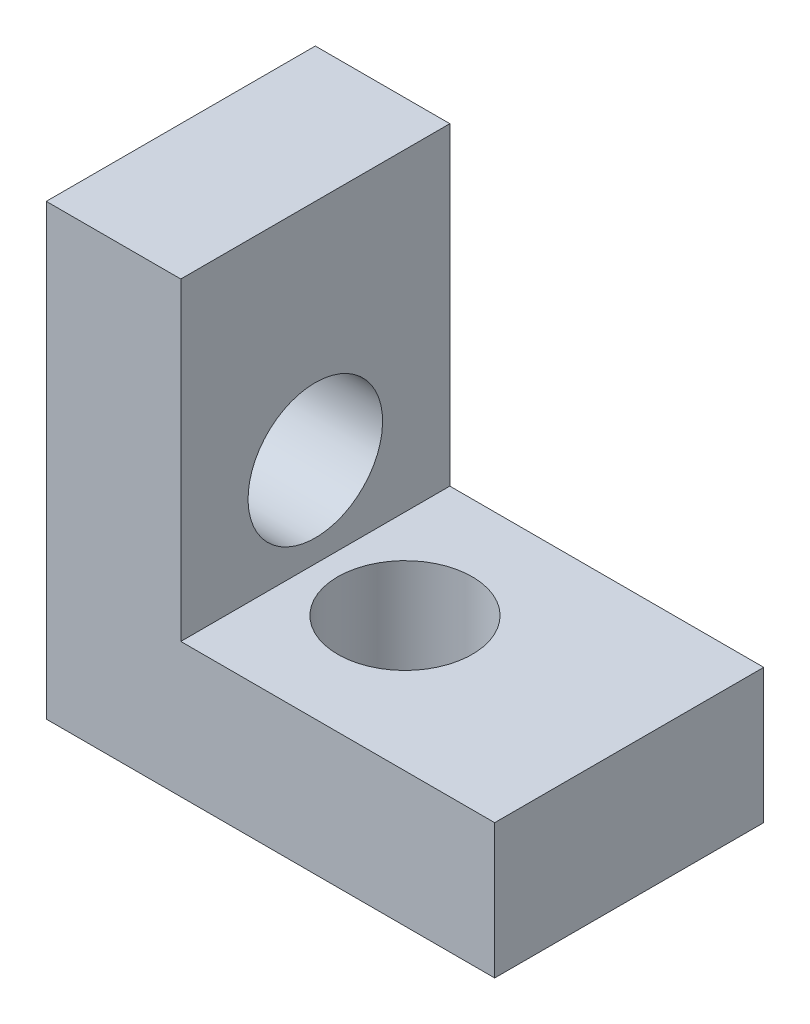
from build123d import *

# Parameters (mm, degrees)
EXTRUDE_4_DEPTH     = 6
SKETCH_7_R          = 1.5
CUT_EXTRUDE_3_DEPTH = 14.601470509
SKETCH_8_R          = 1.5
CUT_EXTRUDE_4_DEPTH = 14.601470509


with BuildPart() as part:
    # 草图6 → 凸台-拉伸4 (new body)
    with BuildSketch(Plane.XY):
        Polygon((0, 0), (10, 0), (10, 3), (3, 3), (3, 10), (0, 10), align=None)
    extrude(amount=EXTRUDE_4_DEPTH)

    # 草图7 → 切除-拉伸3 (cut, through all)
    with BuildSketch(Plane(origin=(3, 0, 0), x_dir=(0, 0, -1), z_dir=(1, 0, 0))):
        with Locations(Location((-3, 5, 0), (0, 0, 90))):
            Circle(SKETCH_7_R)
    extrude(amount=-CUT_EXTRUDE_3_DEPTH, mode=Mode.SUBTRACT)

    # 草图8 → 切除-拉伸4 (cut, through all)
    with BuildSketch(Plane(origin=(0, 3, 0), x_dir=(1, 0, 0), z_dir=(0, 1, 0))):
        with Locations(Location((5, -3, 0), (0, 0, 180))):
            Circle(SKETCH_8_R)
    extrude(amount=-CUT_EXTRUDE_4_DEPTH, mode=Mode.SUBTRACT)


solid = part.part
